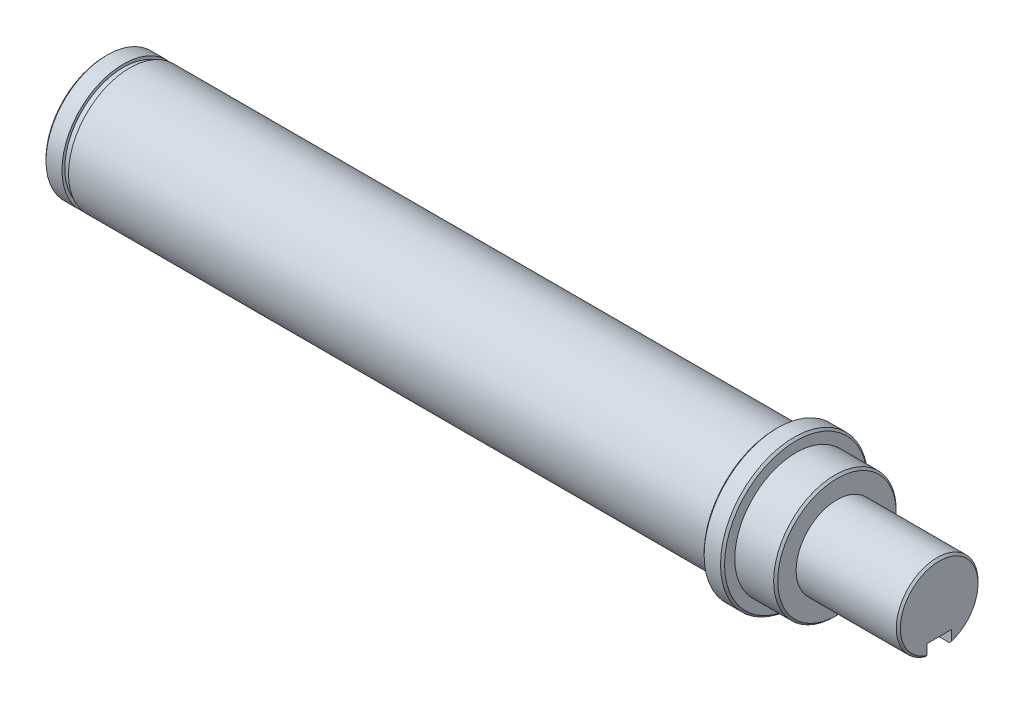
SolidWorks part; units mm, degrees
material "45#"
ref_plane "前基準面" through (0, 0, 0) normal (0, 0, 1) x (1, 0, 0)
ref_plane "上基準面" through (0, 0, 0) normal (0, 1, 0) x (1, 0, 0)
ref_plane "右基準面" through (0, 0, 0) normal (1, 0, 0) x (0, 0, -1)
sketch "草图1" plane through (0, 0, 0) normal (0, 0, 1) x (1, 0, 0)
  line L0 (0, 0) -> (191.287, 0) construction
  line L3 (0, 0) -> (0, 15)
  line L6 (0, 15) -> (4.4, 15)
  line L7 (164, 15) -> (164, 18)
  line L8 (164, 18) -> (169, 18)
  line L9 (169, 18) -> (169, 15)
  line L10 (179, 10) -> (204, 10)
  line L11 (204, 10) -> (204, 0)
  line L12 (204, 0) -> (0, 0)
  line L13 (169, 15) -> (179, 15)
  line L14 (179, 15) -> (179, 10)
  line L15 (4.4, 15) -> (4.4, 14.3)
  line L16 (4.4, 14.3) -> (6, 14.3)
  line L17 (6, 14.3) -> (6, 15)
  line L18 (6, 15) -> (164, 15)
  dimension "D1" = 20
  dimension "D2" = 30
  dimension "D3" = 164
  dimension "D4" = 36
  dimension "D5" = 10
  dimension "D6" = 25
  dimension "D7" = 1.6
  dimension "D8" = 5
  dimension "D9" = 28.6
  dimension "D10" = 6
  dimension "D11" = 4.4
revolve "旋转1" add sketch "草图1" angle 360 about L0
chamfer "倒角1" distance 0.5 angle 45 5 edges at (204, 0, 10) (179, 0, 15) (164, 0, 18) (169, 0, 18) (0, 0, 15)
ref_plane "基准面1" through (0, -15, 0) normal (0, -1, 0) x (-1, 0, 0)
sketch "草图2" plane through (0, -15, 0) normal (0, -1, 0) x (-1, 0, 0)
  line L0 (-49, 0) -> (-119, 0) construction
  line L1 (-49, -4) -> (-119, -4)
  line L2 (-49, 4) -> (-119, 4)
  line L3 (-164, -15) -> (-164, 15) construction
  arc A0 (-49, -4) -> (-49, 4) centre (-49, 0) ccw
  arc A1 (-119, 4) -> (-119, -4) centre (-119, 0) ccw
  point P3 (-84, 0)
  dimension "D1" = 80
  dimension "D2" = 8
  dimension "D3" = 70
extrude "切除-拉伸1" cut sketch "草图2" against normal blind 4
ref_plane "基准面2" through (0, -10, 0) normal (0, -1, 0) x (-1, 0, 0)
sketch "草图3" plane through (0, -10, 0) normal (0, -1, 0) x (-1, 0, 0)
  line L0 (-204, 0) -> (-184, 0) construction
  line L1 (-204, 9.5) -> (-204, -9.5) construction
  line L2 (-204, 3) -> (-184, 3)
  line L3 (-204, -3) -> (-184, -3)
  line L4 (-204, 9.5) -> (-204, -9.5) construction
  arc A0 (-204, 3) -> (-204, -3) centre (-204, 0) ccw
  arc A1 (-184, -3) -> (-184, 3) centre (-184, 0) ccw
  point P4 (-194, 0)
  dimension "D1" = 6
  dimension "D2" = 20
extrude "切除-拉伸2" cut sketch "草图3" against normal blind 3.5
